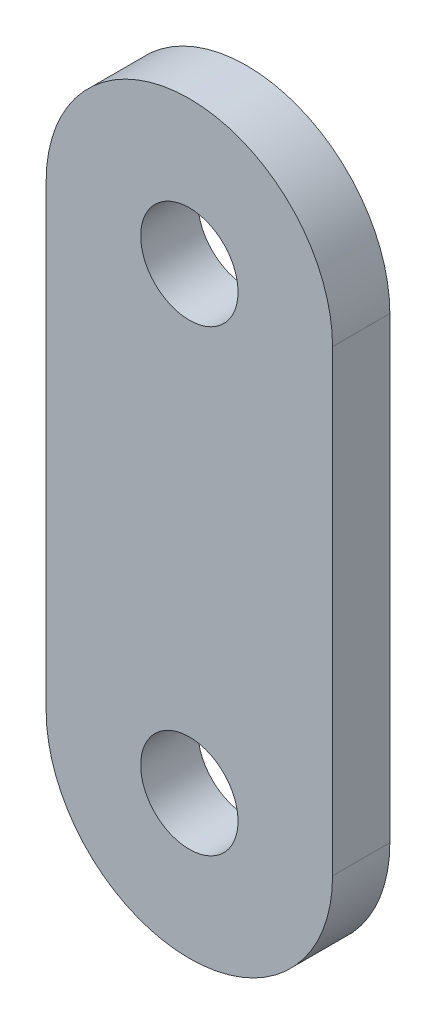
SolidWorks part; units mm, degrees
material "Q235B"
ref_plane "Front Plane" through (0, 0, 0) normal (0, 0, 1) x (1, 0, 0)
ref_plane "Top Plane" through (0, 0, 0) normal (0, 1, 0) x (1, 0, 0)
ref_plane "Right Plane" through (0, 0, 0) normal (1, 0, 0) x (0, 0, -1)
sketch "Sketch1" plane through (0, 0, 0) normal (0, 0, 1) x (1, 0, 0)
  line L0 (0, 0) -> (0, 80) construction
  line L2 (-25, 0) -> (-25, 80)
  line L3 (25, 0) -> (25, 80)
  arc A0 (-25, 0) -> (25, 0) centre (0, 0) ccw
  arc A1 (25, 80) -> (-25, 80) centre (0, 80) ccw
  circle A2 centre (0, 0) radius 8.5
  circle A3 centre (0, 80) radius 8.5
  point P5 (0, 40)
  dimension "D2" = 25
  dimension "D3" = 17
  dimension "D4" = 17
  dimension "D1" = 80
extrude "Boss-Extrude1" add sketch "Sketch1" along normal blind 10
